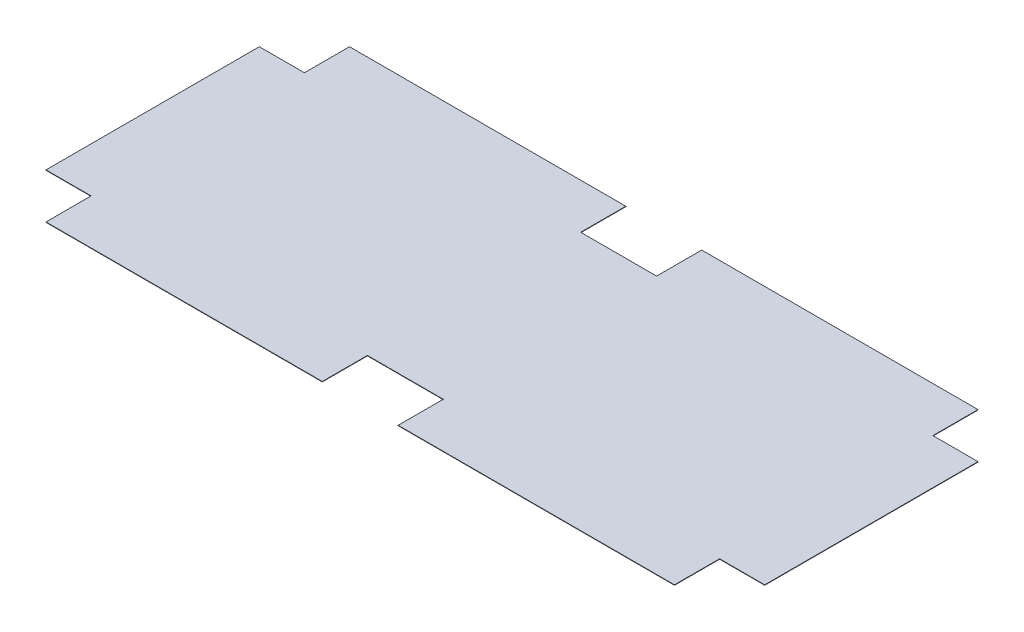
from build123d import *

# Parameters (mm, degrees)
BOSS_EXTRUDE_1_DEPTH = 3


with BuildPart() as part:
    # Sketch 1 → Boss-Extrude 1 (new body)
    with BuildSketch(Plane(origin=(0, 0, 0), x_dir=(1, 0, 0), z_dir=(0, 1, 0))):
        Polygon((2195, 1060), (265, 1060), (265, 745), (-265, 745), (-265, 1060), (-2195, 1060), (-2195, 745), (-2510, 745), (-2510, -745), (-2195, -745), (-2195, -1060), (-265, -1060), (-265, -745), (265, -745), (265, -1060), (2195, -1060), (2195, -745), (2510, -745), (2510, 745), (2195, 745), align=None)
    extrude(amount=BOSS_EXTRUDE_1_DEPTH)


solid = part.part
